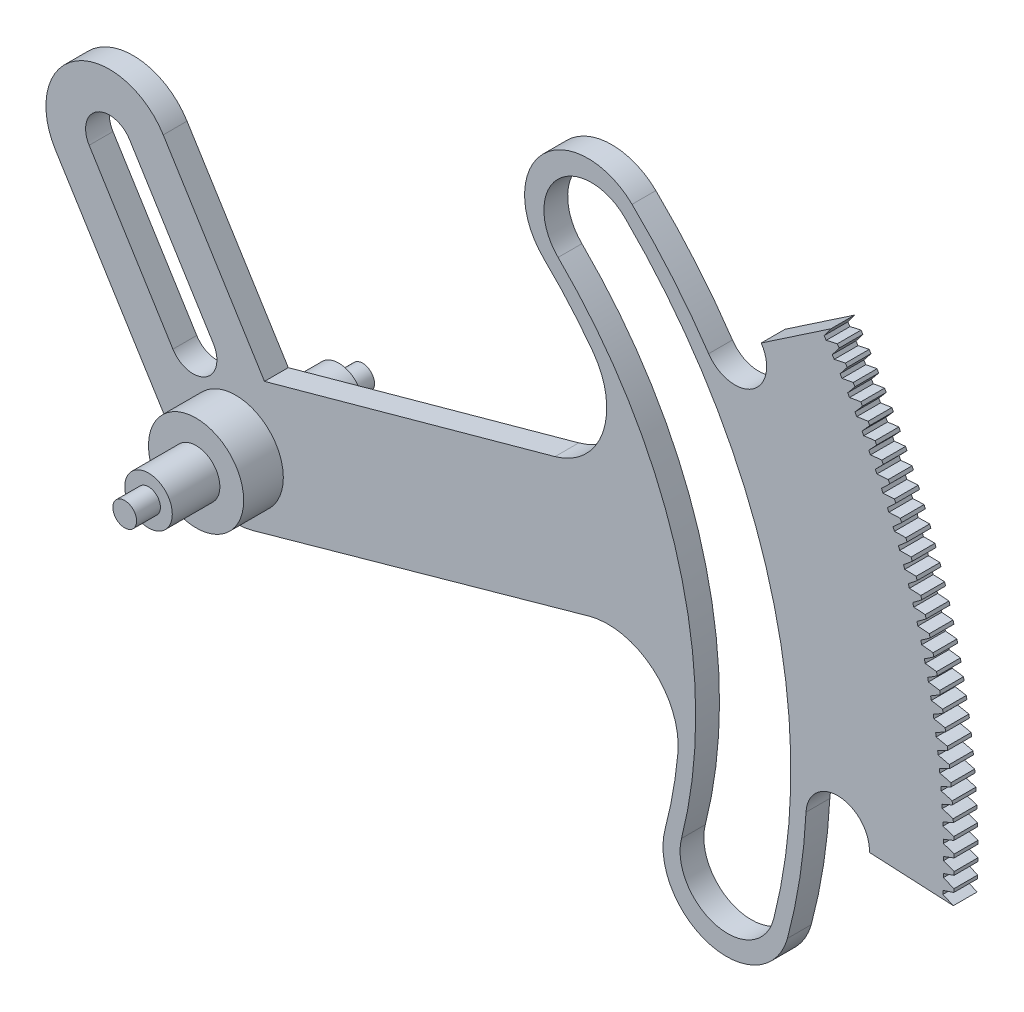
SolidWorks part; units mm, degrees
ref_plane "Front plane" through (0, 0, 0) normal (0, 0, 1) x (1, 0, 0)
ref_plane "Top plane" through (0, 0, 0) normal (0, 1, 0) x (1, 0, 0)
ref_plane "Right plane" through (0, 0, 0) normal (1, 0, 0) x (0, 0, -1)
sketch "Sketch 3" plane through (0, 0, 0) normal (0, 0, 1) x (1, 0, 0)
  line L8 (1.813, 4.66) -> (-4.5702, 14.9275)
  line L9 (-11.3643, 10.7038) -> (-3.3971, -2.1119)
  line L10 (1.0766, -3.8524) -> (22.2647, 2.0692)
  line L12 (0, 0) -> (66.0533, 18.4603) construction
  line L14 (-6.6933, 13.6076) -> (-1.4136, 5.115)
  line L15 (-9.2411, 12.0237) -> (-3.9614, 3.5311)
  line L17 (1.813, 4.66) -> (20.1291, 9.7107)
  line L18 (22.2647, 2.0692) -> (20.1291, 9.7107) construction
  line L19 (27.0692, -7.1593) -> (19.4352, 20.1562) construction
  line L20 (28.1049, -7.1496) -> (20.3258, 20.6848) construction
  arc A12 (-4.5702, 14.9275) -> (-11.3643, 10.7038) centre (-7.9672, 12.8157) ccw
  arc A13 (-3.3971, -2.1119) -> (1.0766, -3.8524) centre (0, 0) ccw
  arc A18 (-6.6933, 13.6076) -> (-9.2411, 12.0237) centre (-7.9672, 12.8157) ccw
  arc A19 (-3.9614, 3.5311) -> (-1.4136, 5.115) centre (-2.6875, 4.323) ccw
  circle A23 centre (0, 0) radius 32 construction
  arc A24 (27.0692, -7.1593) -> (27.8772, -2.6197) centre (0, 0) ccw
  arc A25 (34.7865, -9.2681) -> (24.9881, 25.9151) centre (0, 0) ccw
  arc A26 (22.2647, 2.0692) -> (27.8772, -2.6197) centre (23.4591, -2.2046) cw
  arc A27 (20.1291, 9.7107) -> (22.5225, 16.6354) centre (18.9477, 13.995) ccw
  arc A28 (27.0692, -7.1593) -> (34.7865, -9.2681) centre (30.9365, -8.1822) ccw
  arc A29 (19.4352, 20.1562) -> (24.9881, 25.9151) centre (22.2117, 23.0357) cw
  arc A30 (28.1049, -7.1496) -> (20.3258, 20.6848) centre (0, 0) ccw
  arc A31 (33.9197, -8.6289) -> (24.5311, 24.9644) centre (0, 0) ccw
  arc A32 (28.1049, -7.1496) -> (33.9197, -8.6289) centre (31.0123, -7.8892) ccw
  arc A33 (20.3258, 20.6848) -> (24.5311, 24.9644) centre (22.4285, 22.8246) cw
  arc A34 (22.5225, 16.6354) -> (19.4352, 20.1562) centre (0, 0) ccw
  point P16 (23.9756, 17.8783)
  point P20 (27.0692, -7.1593)
  point P22 (29.7842, -2.471)
  point P38 (27.8495, -8.0875)
  dimension "D1" = 3
  dimension "D2" = 4
  dimension "D5" = 12.09
  dimension "D7" = 64
  dimension "D11" = 22
  dimension "D12" = 4
  dimension "D13" = 1
  dimension "D15" = 70
  dimension "D9" = 56
  dimension "D10" = 72
  dimension "D8" = 2
  dimension "D14" = 58
  dimension "D3" = 10
  dimension "D4" = 10
  dimension "D6" = 15.0903
sketch "Sketch 6" plane through (0, 0, 0) normal (0, 0, 1) x (1, 0, 0)
  line L8 (0, 0) -> (52.129, 14.5688) construction
  line L17 (37.5198, 25.3842) -> (33.13, 22.4143)
  line L18 (39.9505, -1.99) -> (45.2439, -2.2537)
  line L19 (42.9772, 12.0111) -> (0, 0) construction
  arc A157 (45.2986, -0.3571) -> (44.6239, -0.1057) centre (38.6767, -17.0948) ccw
  arc A158 (44.6239, -0.1057) -> (44.6238, 0.1281) centre (0, 0) ccw
  arc A159 (44.6238, 0.1281) -> (45.2984, 0.3799) centre (38.6681, 17.1143) ccw
  arc A160 (45.2984, 0.3799) -> (45.2961, 0.5916) centre (0, 0) ccw
  arc A161 (45.2961, 0.5916) -> (44.6163, 0.8289) centre (39.0262, -16.2811) ccw
  arc A162 (44.6163, 0.8289) -> (44.6113, 1.0626) centre (0, 0) ccw
  arc A163 (44.6113, 1.0626) -> (45.2805, 1.3285) centre (38.3012, 17.9203) ccw
  arc A164 (45.2805, 1.3285) -> (45.2738, 1.5401) centre (0, 0) ccw
  arc A165 (45.2738, 1.5401) -> (44.5892, 1.7631) centre (39.3586, -15.4602) ccw
  arc A166 (44.5892, 1.7631) -> (44.5793, 1.9966) centre (0, 0) ccw
  arc A167 (44.5793, 1.9966) -> (45.2428, 2.2765) centre (37.9175, 18.7185) ccw
  arc A168 (45.2428, 2.2765) -> (45.2316, 2.4879) centre (0, 0) ccw
  arc A169 (45.2316, 2.4879) -> (44.5425, 2.6965) centre (39.6738, -14.6326) ccw
  arc A170 (44.5425, 2.6965) -> (44.5277, 2.9298) centre (0, 0) ccw
  arc A171 (44.5277, 2.9298) -> (45.1852, 3.2234) centre (37.5172, 19.5085) ccw
  arc A172 (45.1852, 3.2234) -> (45.1696, 3.4346) centre (0, 0) ccw
  arc A173 (45.1696, 3.4346) -> (44.4762, 3.6287) centre (39.9715, -13.7985) ccw
  arc A174 (44.4762, 3.6287) -> (44.4566, 3.8617) centre (0, 0) ccw
  arc A175 (44.4566, 3.8617) -> (45.1078, 4.169) centre (37.1004, 20.2899) ccw
  arc A176 (45.1078, 4.169) -> (45.0878, 4.3798) centre (0, 0) ccw
  arc A177 (45.0878, 4.3798) -> (44.3905, 4.5594) centre (40.2517, -12.9584) ccw
  arc A178 (44.3905, 4.5594) -> (44.366, 4.7919) centre (0, 0) ccw
  arc A179 (44.366, 4.7919) -> (45.0105, 5.1128) centre (36.6673, 21.0624) ccw
  arc A180 (45.0105, 5.1128) -> (44.9862, 5.3231) centre (0, 0) ccw
  arc A181 (44.9862, 5.3231) -> (44.2852, 5.488) centre (40.5143, -12.1126) ccw
  arc A182 (44.2852, 5.488) -> (44.2559, 5.7199) centre (0, 0) ccw
  arc A183 (44.2559, 5.7199) -> (44.8936, 6.0543) centre (36.2182, 21.8257) ccw
  arc A184 (44.8936, 6.0543) -> (44.8648, 6.2641) centre (0, 0) ccw
  arc A185 (44.8648, 6.2641) -> (44.1606, 6.4142) centre (40.759, -11.2614) ccw
  arc A186 (44.1606, 6.4142) -> (44.1264, 6.6455) centre (0, 0) ccw
  arc A187 (44.1264, 6.6455) -> (44.757, 6.9931) centre (35.7532, 22.5794) ccw
  arc A188 (44.757, 6.9931) -> (44.7238, 7.2023) centre (0, 0) ccw
  arc A189 (44.7238, 7.2023) -> (44.0166, 7.3377) centre (40.986, -10.4054) ccw
  arc A190 (44.0166, 7.3377) -> (43.9775, 7.5682) centre (0, 0) ccw
  arc A191 (43.9775, 7.5682) -> (44.6007, 7.9289) centre (35.2725, 23.3232) ccw
  arc A192 (44.6007, 7.9289) -> (44.5631, 8.1373) centre (0, 0) ccw
  arc A193 (44.5631, 8.1373) -> (43.8533, 8.2579) centre (41.1949, -9.5447) ccw
  arc A194 (43.8533, 8.2579) -> (43.8094, 8.4875) centre (0, 0) ccw
  arc A195 (43.8094, 8.4875) -> (44.4249, 8.8612) centre (34.7763, 24.0568) ccw
  arc A196 (44.4249, 8.8612) -> (44.383, 9.0688) centre (0, 0) ccw
  arc A197 (44.383, 9.0688) -> (43.6707, 9.1745) centre (41.3857, -8.6799) ccw
  arc A198 (43.6707, 9.1745) -> (43.622, 9.4031) centre (0, 0) ccw
  arc A199 (43.622, 9.4031) -> (44.2295, 9.7897) centre (34.2649, 24.7798) ccw
  arc A200 (44.2295, 9.7897) -> (44.1833, 9.9963) centre (0, 0) ccw
  arc A201 (44.1833, 9.9963) -> (43.469, 10.087) centre (41.5584, -7.8113) ccw
  arc A202 (43.469, 10.087) -> (43.4156, 10.3146) centre (0, 0) ccw
  arc A203 (43.4156, 10.3146) -> (44.0148, 10.7138) centre (33.7384, 25.492) ccw
  arc A204 (44.0148, 10.7138) -> (43.9643, 10.9194) centre (0, 0) ccw
  arc A205 (43.9643, 10.9194) -> (43.2482, 10.9951) centre (41.7129, -6.9393) ccw
  arc A206 (43.2482, 10.9951) -> (43.19, 11.2216) centre (0, 0) ccw
  arc A207 (43.19, 11.2216) -> (43.7808, 11.6332) centre (33.1971, 26.1929) ccw
  arc A208 (43.7808, 11.6332) -> (43.7259, 11.8377) centre (0, 0) ccw
  arc A209 (43.7259, 11.8377) -> (43.0085, 11.8985) centre (41.8491, -6.0642) ccw
  arc A210 (43.0085, 11.8985) -> (42.9455, 12.1236) centre (0, 0) ccw
  arc A211 (42.9455, 12.1236) -> (43.5276, 12.5475) centre (32.6413, 26.8824) ccw
  arc A212 (43.5276, 12.5475) -> (43.4684, 12.7508) centre (0, 0) ccw
  arc A213 (43.4684, 12.7508) -> (42.7499, 12.7965) centre (41.9669, -5.1864) ccw
  arc A214 (42.7499, 12.7965) -> (42.6822, 13.0203) centre (0, 0) ccw
  arc A215 (42.6822, 13.0203) -> (43.2552, 13.4564) centre (32.0712, 27.5601) ccw
  arc A216 (43.2552, 13.4564) -> (43.1919, 13.6584) centre (0, 0) ccw
  arc A217 (43.1919, 13.6584) -> (42.4725, 13.689) centre (42.0663, -4.3064) ccw
  arc A218 (42.4725, 13.689) -> (42.4002, 13.9113) centre (0, 0) ccw
  arc A219 (42.4002, 13.9113) -> (42.964, 14.3593) centre (31.487, 28.2257) ccw
  arc A220 (42.964, 14.3593) -> (42.8964, 14.5599) centre (0, 0) ccw
  arc A221 (42.8964, 14.5599) -> (42.1765, 14.5755) centre (42.1473, -3.4245) ccw
  arc A222 (42.1765, 14.5755) -> (42.0996, 14.7963) centre (0, 0) ccw
  arc A223 (42.0996, 14.7963) -> (42.6538, 15.2559) centre (30.8889, 28.8789) ccw
  arc A224 (42.6538, 15.2559) -> (42.582, 15.4551) centre (0, 0) ccw
  arc A225 (42.582, 15.4551) -> (41.862, 15.4556) centre (42.2098, -2.5411) ccw
  arc A226 (41.862, 15.4556) -> (41.7804, 15.6747) centre (0, 0) ccw
  arc A227 (41.7804, 15.6747) -> (42.325, 16.1458) centre (30.2774, 29.5195) ccw
  arc A228 (42.325, 16.1458) -> (42.249, 16.3435) centre (0, 0) ccw
  arc A229 (42.249, 16.3435) -> (41.5291, 16.3289) centre (42.2537, -1.6565) ccw
  arc A230 (41.5291, 16.3289) -> (41.443, 16.5462) centre (0, 0) ccw
  arc A231 (41.443, 16.5462) -> (41.9775, 17.0287) centre (29.6525, 30.1471) ccw
  arc A232 (41.9775, 17.0287) -> (41.8975, 17.2247) centre (0, 0) ccw
  arc A233 (41.8975, 17.2247) -> (41.1781, 17.195) centre (42.2791, -0.7713) ccw
  arc A234 (41.1781, 17.195) -> (41.0874, 17.4105) centre (0, 0) ccw
  arc A235 (41.0874, 17.4105) -> (41.6117, 17.904) centre (29.0147, 30.7615) ccw
  arc A236 (41.6117, 17.904) -> (41.5276, 18.0983) centre (0, 0) ccw
  arc A237 (41.5276, 18.0983) -> (40.8089, 18.0536) centre (42.286, 0.1143) ccw
  arc A238 (40.8089, 18.0536) -> (40.7138, 18.2672) centre (0, 0) ccw
  arc A239 (40.7138, 18.2672) -> (41.2276, 18.7716) centre (28.3641, 31.3624) ccw
  arc A240 (41.2276, 18.7716) -> (41.1395, 18.9641) centre (0, 0) ccw
  arc A241 (41.1395, 18.9641) -> (40.4219, 18.9043) centre (42.2743, 0.9999) ccw
  arc A242 (40.4219, 18.9043) -> (40.3223, 19.1158) centre (0, 0) ccw
  arc A243 (40.3223, 19.1158) -> (40.8255, 19.6309) centre (27.7011, 31.9495) ccw
  arc A244 (40.8255, 19.6309) -> (40.7333, 19.8215) centre (0, 0) ccw
  arc A245 (40.7333, 19.8215) -> (40.0171, 19.7467) centre (42.2441, 1.885) ccw
  arc A246 (40.0171, 19.7467) -> (39.9131, 19.9561) centre (0, 0) ccw
  arc A247 (39.9131, 19.9561) -> (40.4054, 20.4815) centre (27.0259, 32.5226) ccw
  arc A248 (40.4054, 20.4815) -> (40.3092, 20.6702) centre (0, 0) ccw
  arc A249 (40.3092, 20.6702) -> (39.5948, 20.5804) centre (42.1954, 2.7693) ccw
  arc A250 (39.5948, 20.5804) -> (39.4864, 20.7876) centre (0, 0) ccw
  arc A251 (39.4864, 20.7876) -> (39.9676, 21.3232) centre (26.3388, 33.0815) ccw
  arc A252 (39.9676, 21.3232) -> (39.8675, 21.5098) centre (0, 0) ccw
  arc A253 (39.8675, 21.5098) -> (39.1551, 21.4051) centre (42.1281, 3.6523) ccw
  arc A254 (39.1551, 21.4051) -> (39.0424, 21.6099) centre (0, 0) ccw
  arc A255 (39.0424, 21.6099) -> (39.5123, 22.1556) centre (25.6403, 33.6258) ccw
  arc A256 (39.5123, 22.1556) -> (39.4083, 22.34) centre (0, 0) ccw
  arc A257 (39.4083, 22.34) -> (38.6983, 22.2204) centre (42.0424, 4.5338) ccw
  arc A258 (38.6983, 22.2204) -> (38.5813, 22.4228) centre (0, 0) ccw
  arc A259 (38.5813, 22.4228) -> (39.0396, 22.9782) centre (24.9304, 34.1554) ccw
  arc A260 (39.0396, 22.9782) -> (38.9318, 23.1604) centre (0, 0) ccw
  arc A261 (38.9318, 23.1604) -> (38.2244, 23.026) centre (41.9382, 5.4133) ccw
  arc A262 (38.2244, 23.026) -> (38.1033, 23.2259) centre (0, 0) ccw
  arc A263 (38.1033, 23.2259) -> (38.5498, 23.7907) centre (24.2097, 34.67) ccw
  arc A264 (38.5498, 23.7907) -> (38.4382, 23.9707) centre (0, 0) ccw
  arc A265 (38.4382, 23.9707) -> (37.7338, 23.8214) centre (41.8157, 6.2904) ccw
  arc A266 (37.7338, 23.8214) -> (37.6085, 24.0188) centre (0, 0) ccw
  arc A267 (37.6085, 24.0188) -> (38.0432, 24.5928) centre (23.4783, 35.1694) ccw
  arc A268 (38.0432, 24.5928) -> (37.9278, 24.7704) centre (0, 0) ccw
  arc A269 (37.9278, 24.7704) -> (37.2267, 24.6064) centre (41.6748, 7.1647) ccw
  arc A270 (37.2267, 24.6064) -> (37.0972, 24.8011) centre (0, 0) ccw
  arc A271 (37.0972, 24.8011) -> (37.5198, 25.3842) centre (22.7366, 35.6534) ccw
  arc A273 (45.2439, -2.2537) -> (44.5803, -1.9742) centre (37.9269, -18.6994) ccw
  arc A274 (44.5803, -1.9742) -> (44.59, -1.7407) centre (0, 0) ccw
  arc A275 (44.59, -1.7407) -> (45.2746, -1.5173) centre (39.3509, 15.48) ccw
  arc A276 (45.2746, -1.5173) -> (45.2812, -1.3057) centre (0, 0) ccw
  arc A277 (45.2812, -1.3057) -> (44.6119, -1.0402) centre (38.3102, -17.9011) ccw
  arc A278 (44.6119, -1.0402) -> (44.6167, -0.8065) centre (0, 0) ccw
  arc A279 (44.6167, -0.8065) -> (45.2964, -0.5689) centre (39.018, 16.3007) ccw
  arc A280 (45.2964, -0.5689) -> (45.2986, -0.3571) centre (0, 0) ccw
  arc A282 (35.9554, -1.791) -> (29.817, 20.1729) centre (0, 0) ccw
  arc A284 (29.817, 20.1729) -> (33.13, 22.4143) centre (31.4735, 21.2936) ccw
  arc A286 (35.9554, -1.791) -> (39.9505, -1.99) centre (37.9529, -1.8905) cw
  point P0 (42.9772, 12.0111)
  point P3 (16.556, 4.627)
  dimension "D2" = 72
  dimension "D1" = 2
  dimension "D3" = 2
extrude "Boss-Extrude 2" add sketch "Sketch 6" along normal blind 1.5
extrude "Boss-Extrude 3" add sketch "Sketch 3" along normal blind 1.5
sketch "Sketch 12" plane through (0, 0, 1.5) normal (0, 0, 1) x (1, 0, 0)
  circle A0 centre (0, 0) radius 3
  dimension "D1" = 6
extrude "Boss-Extrude 4" add sketch "Sketch 12" along normal blind 2.5
sketch "Sketch 13" plane through (0, 0, 4) normal (0, 0, 1) x (1, 0, 0)
  circle A0 centre (0, 0) radius 1.5
  dimension "D1" = 3
extrude "Boss-Extrude 5" add sketch "Sketch 13" along normal blind 3
sketch "Sketch 14" plane through (0, 0, 7) normal (0, 0, 1) x (1, 0, 0)
  circle A0 centre (0, 0) radius 0.75
  dimension "D1" = 1.5
extrude "Boss-Extrude 6" add sketch "Sketch 14" along normal blind 1.5
sketch "Sketch 15" plane through (0, 0, 0) normal (0, 0, -1) x (-1, 0, 0)
  circle A0 centre (0, 0) radius 1.5
  dimension "D1" = 3
extrude "Boss-Extrude 7" add sketch "Sketch 15" along normal blind 5
sketch "Sketch 16" plane through (0, 0, -5) normal (0, 0, -1) x (-1, 0, 0)
  circle A0 centre (0, 0) radius 0.75
  dimension "D1" = 1.5
extrude "Boss-Extrude 8" add sketch "Sketch 16" along normal blind 1.5
